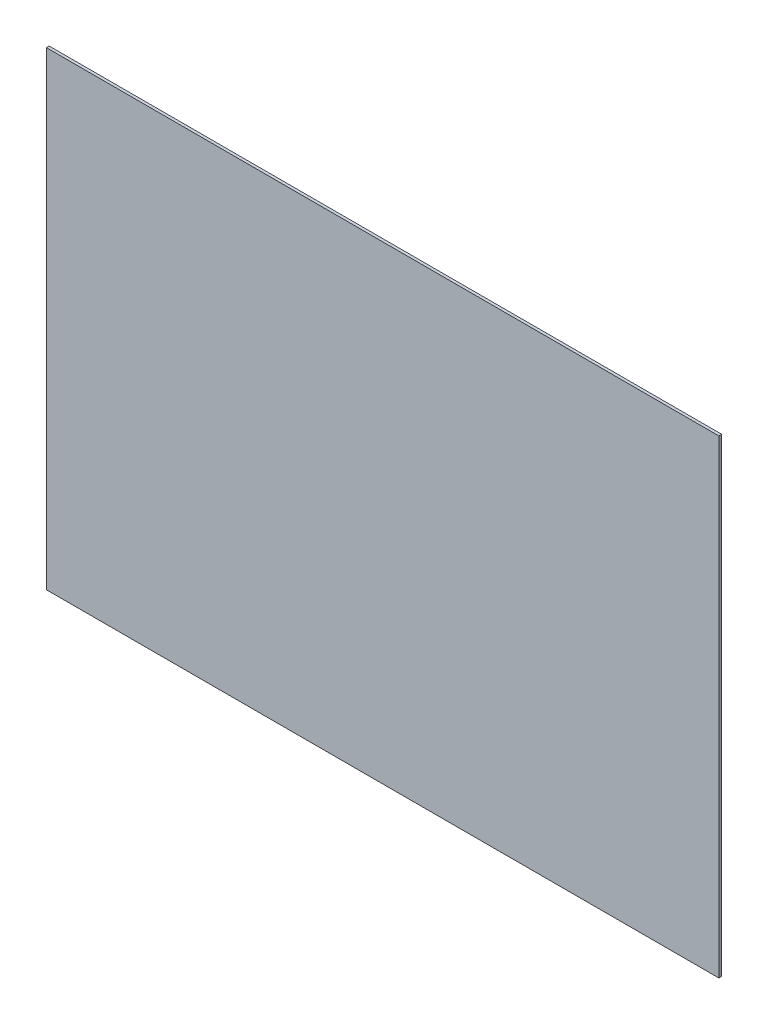
SolidWorks part; units mm, degrees
material "PMMA(有机玻璃)"
ref_plane "前视" through (0, 0, 0) normal (0, 0, 1) x (1, 0, 0)
ref_plane "上视" through (0, 0, 0) normal (0, 1, 0) x (1, 0, 0)
ref_plane "右视" through (0, 0, 0) normal (1, 0, 0) x (0, 0, -1)
sketch "草图1" plane through (0, 0, 0) normal (0, 0, 1) x (1, 0, 0)
  line L1 (-603, 421) -> (603, 421)
  line L2 (-603, 421) -> (-603, -421)
  line L3 (-603, -421) -> (603, -421)
  line L4 (603, 421) -> (603, -421)
  line L5 (-603, 421) -> (603, -421) construction
  line L6 (-603, -421) -> (603, 421) construction
  point P0 (0, 0)
  dimension "D1" = 842
  dimension "D2" = 1206
extrude "凸台-拉伸1" add sketch "草图1" along normal blind 5
hole_wizard "M5 间隙孔1" positions "草图3" profile "草图2" hole size "M5" standard "GB"
sketch "草图3" plane through (0, 0, 5) normal (0, 0, 1) x (1, 0, 0)
  line L0 (-427.5, 273) -> (-427.5, -273) construction
  line L1 (-427.5, -273) -> (427.5, -273) construction
  line L2 (0, 273) -> (0, -273) construction
  line L3 (427.5, 273) -> (-427.5, 273) construction
  line L5 (-427.5, 0) -> (427.5, 0) construction
  line L6 (427.5, -273) -> (427.5, 273) construction
  point P0 (-375, -261)
  point P46 (415.5, 250)
  point P48 (-415.5, 250)
  point P58 (-125, -261)
  point P59 (125, -261)
  point P61 (-125, 261)
  point P62 (125, 261)
  point P64 (-375, 261)
  point P88 (375, -261)
  point P89 (375, 261)
  point P108 (415.5, 0)
  point P109 (-415.5, 0)
  point P110 (415.5, -250)
  point P111 (-415.5, -250)
  dimension "D1" = 12
  dimension "D2" = 12
  dimension "D5" = 3
  dimension "D3" = 12
  dimension "D6" = 4
  dimension "D4" = 2
sketch "草图2" plane through (-375, -261, 5) normal (1, 0, 0) x (0, -1, 0)
  line L0 (0, 0) -> (0, 5)
  line L1 (0, 5) -> (2.75, 5)
  line L2 (2.75, 5) -> (2.75, 0)
  line L5 (2.75, 0) -> (0, 0)
  line L11 (0, -6.35) -> (0, 107.95) construction
  dimension "通孔孔直径" = 5.5
  dimension "通孔孔深度" = 5
